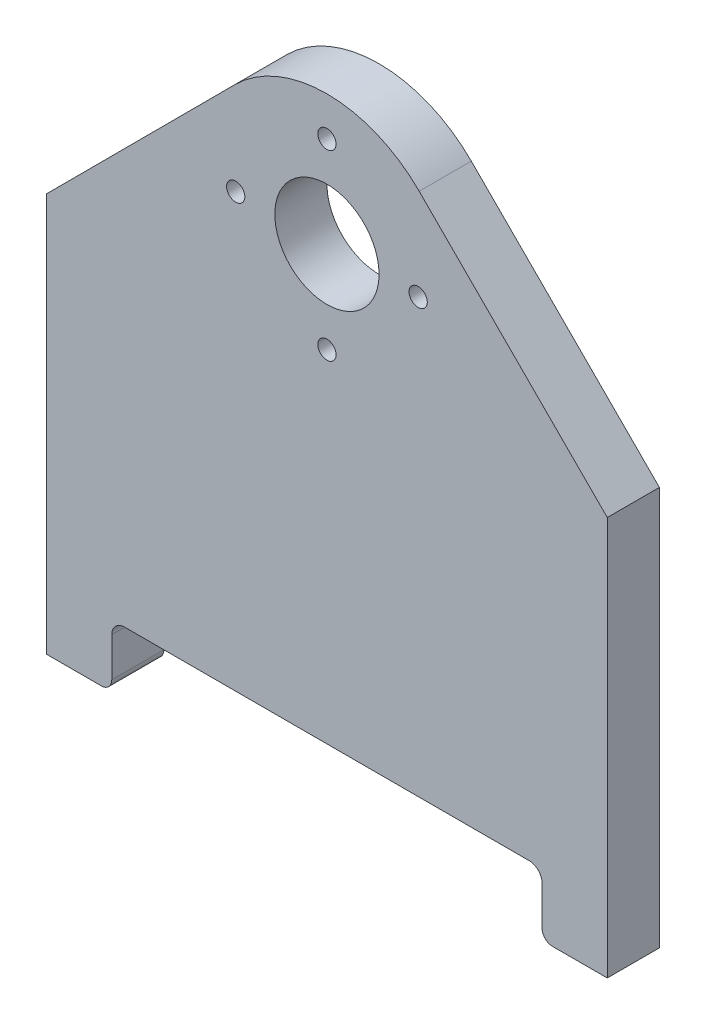
from build123d import *

# Parameters (mm, degrees)
SKETCH1_R           = 40
BOSS_EXTRUDE1_DEPTH = 40
M16_TAPPED_HOLE1_D  = 14


with BuildPart() as part:
    # Sketch1 → Boss-Extrude1 (new body)
    with BuildSketch(Plane.XY):
        with BuildLine():
            Line((-215.1, -380), (-173.1, -380))
            ThreePointArc((-173.1, -380), (-167.443145751, -377.656854249), (-165.1, -372))
            Line((-165.1, -372), (-165.1, -342))
            ThreePointArc((-165.1, -342), (-162.171067812, -334.928932188), (-155.1, -332))
            Line((-155.1, -332), (155.1, -332))
            ThreePointArc((155.1, -332), (162.171067812, -334.928932188), (165.1, -342))
            Line((165.1, -342), (165.1, -372))
            ThreePointArc((165.1, -372), (167.443145751, -377.656854249), (173.1, -380))
            Line((173.1, -380), (215.1, -380))
            Line((215.1, -380), (215.1, -74))
            Line((215.1, -74), (70.789255941, 70.632012878))
            ThreePointArc((70.789255941, 70.632012878), (0, 100), (-70.789255941, 70.632012878))
            Line((-70.789255941, 70.632012878), (-215.1, -74))
            Line((-215.1, -74), (-215.1, -380))
        make_face()
        Circle(SKETCH1_R, mode=Mode.SUBTRACT)
    extrude(amount=BOSS_EXTRUDE1_DEPTH)

    # M16 Tapped Hole1 (through all)
    with Locations(Plane.XY.offset(40)):
        with Locations((0, 70), (70, 0), (0, -70), (-70, 0)):
            Hole(M16_TAPPED_HOLE1_D / 2)


solid = part.part
